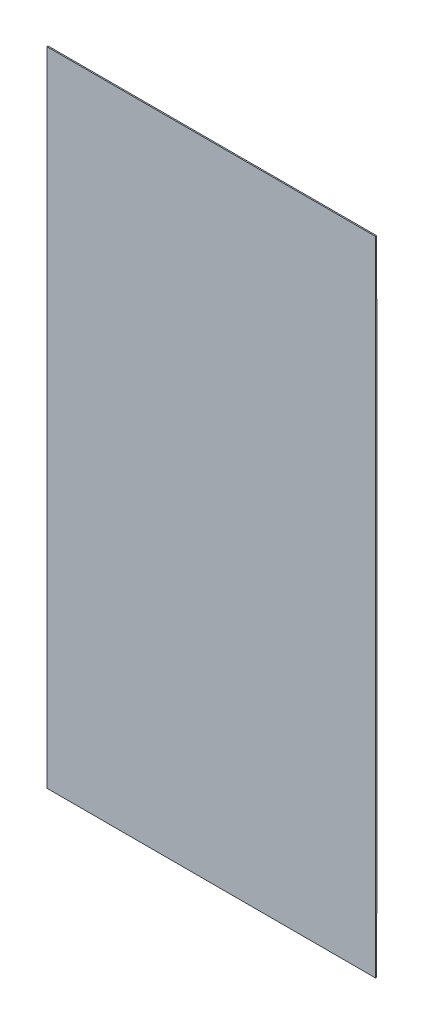
from build123d import *

# Parameters (mm, degrees)
SKETCH_1_W      = 1100
SKETCH_1_H      = 2150
EXTRUDE_1_DEPTH = 4
SKETCH_2_W      = 1100
SKETCH_2_H      = 1780
EXTRUDE_2_DEPTH = 1


with BuildPart() as part:
    # 草图1 → 凸台-拉伸1 (new body)
    with BuildSketch(Plane.XY):
        with Locations((550, -1075)):
            Rectangle(SKETCH_1_W, SKETCH_1_H)
    extrude(amount=EXTRUDE_1_DEPTH)

    # 草图2 → 凸台-拉伸2 (add)
    with BuildSketch(Plane(origin=(0, 0, 0), x_dir=(-1, 0, 0), z_dir=(0, 0, -1))):
        with Locations((-550, -1075)):
            Rectangle(SKETCH_2_W, SKETCH_2_H)
    extrude(amount=EXTRUDE_2_DEPTH)


solid = part.part
